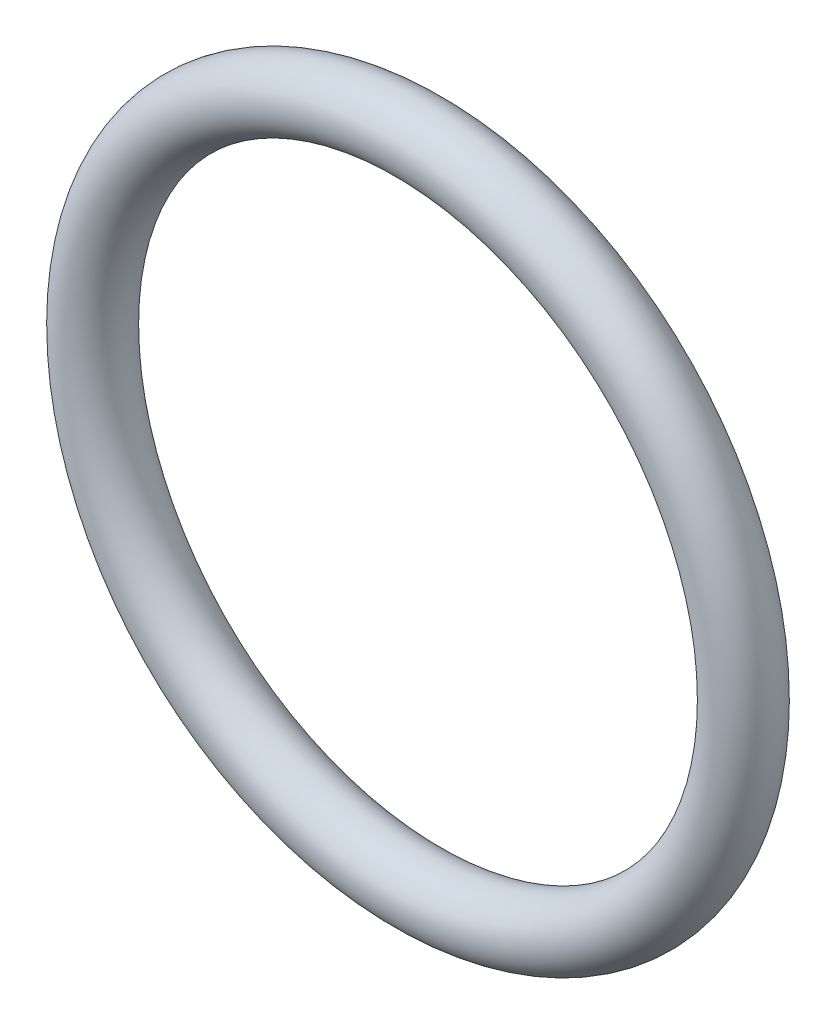
from build123d import *

# Parameters (mm, degrees)
SKETCH1_R = 1


with BuildPart() as part:
    # Sketch1 → Revolve1 (revolve)
    with BuildSketch(Plane(origin=(0, 0, 0), x_dir=(1, 0, 0), z_dir=(0, 1, 0)), mode=Mode.PRIVATE) as revolve1_sk:
        with Locations((10, 0)):
            Circle(SKETCH1_R)
    revolve(revolve1_sk.sketch.rotate(Axis((0, 0, 0), (0, 0, 1)), 180), axis=Axis((0, 0, 0), (0, 0, 1)))


solid = part.part
